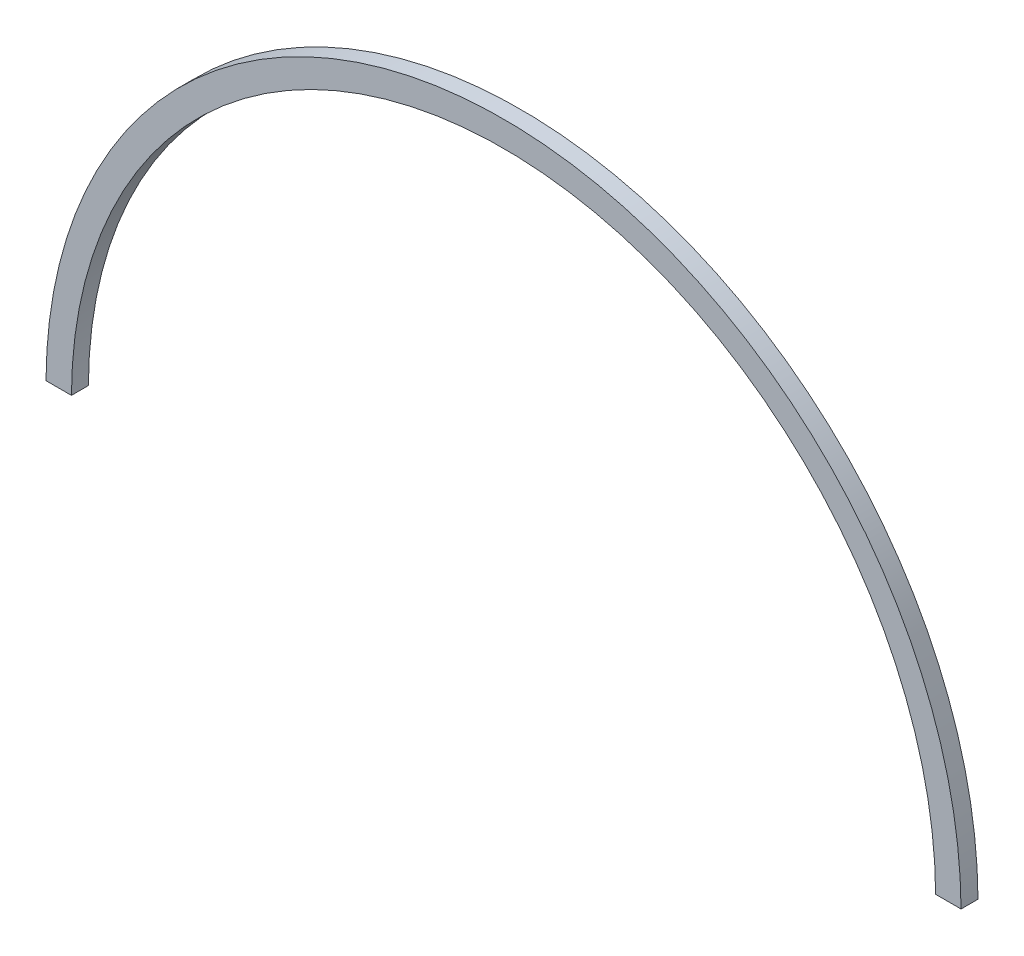
from build123d import *

# Parameters (mm, degrees)
EXTRUDE_1_DEPTH = 4


with BuildPart() as part:
    # 草图1 → 凸台-拉伸1 (new, symmetric)
    with BuildSketch(Plane.XY):
        with BuildLine():
            Line((4.002314827, 1), (16.002450995, 1))
            ThreePointArc((16.002450995, 1), (220, 204), (423.997549005, 1))
            Line((423.997549005, 1), (435.997685173, 1))
            ThreePointArc((435.997685173, 1), (220, 216), (4.002314827, 1))
        make_face()
    extrude(amount=EXTRUDE_1_DEPTH, both=True)


solid = part.part
